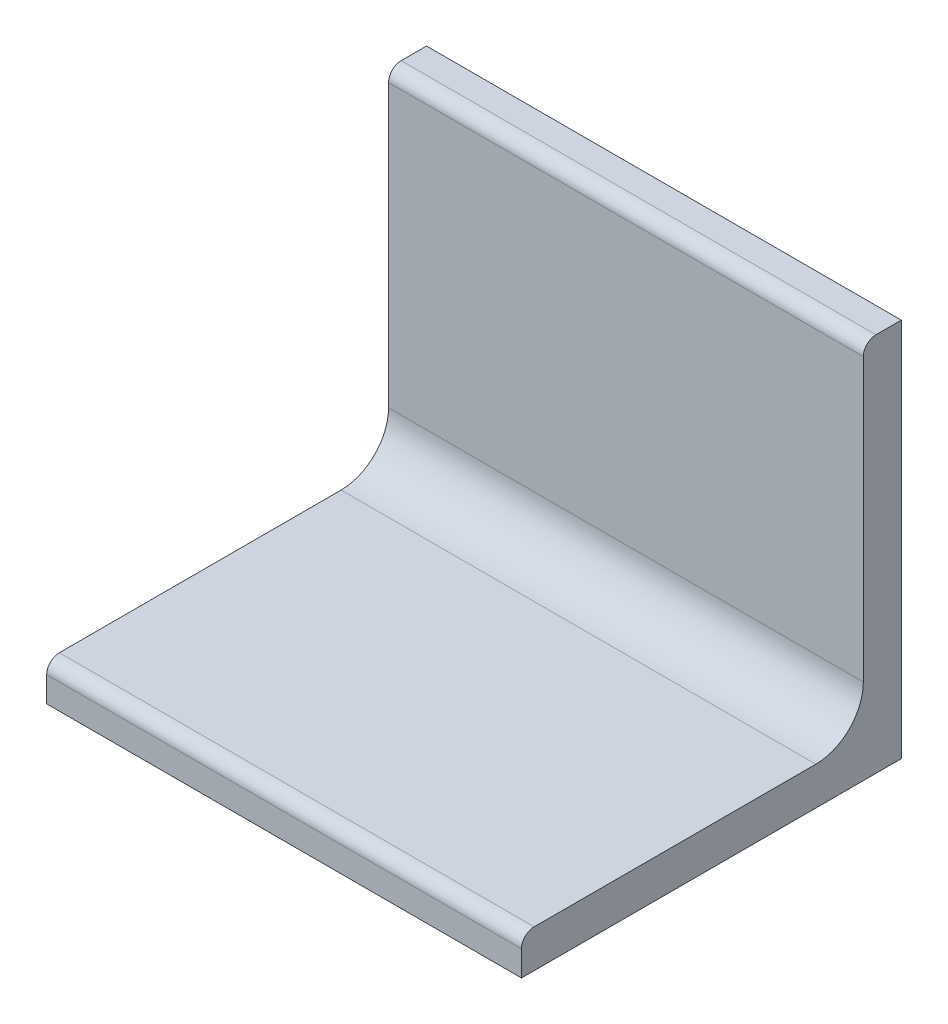
from build123d import *

# Parameters (mm, degrees)
BASE_DEPTH = 50


with BuildPart() as part:
    # Sketch1 → Base (new body)
    with BuildSketch(Plane.YZ):
        with BuildLine():
            Line((0, 40), (0, 0))
            Line((0, 0), (40, 0))
            Line((40, 0), (40, 2.666666667))
            ThreePointArc((40, 2.666666667), (39.609475708, 3.609475708), (38.666666667, 4))
            Line((38.666666667, 4), (9, 4))
            ThreePointArc((9, 4), (5.464466094, 5.464466094), (4, 9))
            Line((4, 9), (4, 38.666666667))
            ThreePointArc((4, 38.666666667), (3.609475708, 39.609475708), (2.666666667, 40))
            Line((2.666666667, 40), (0, 40))
        make_face()
    extrude(amount=BASE_DEPTH)


solid = part.part
